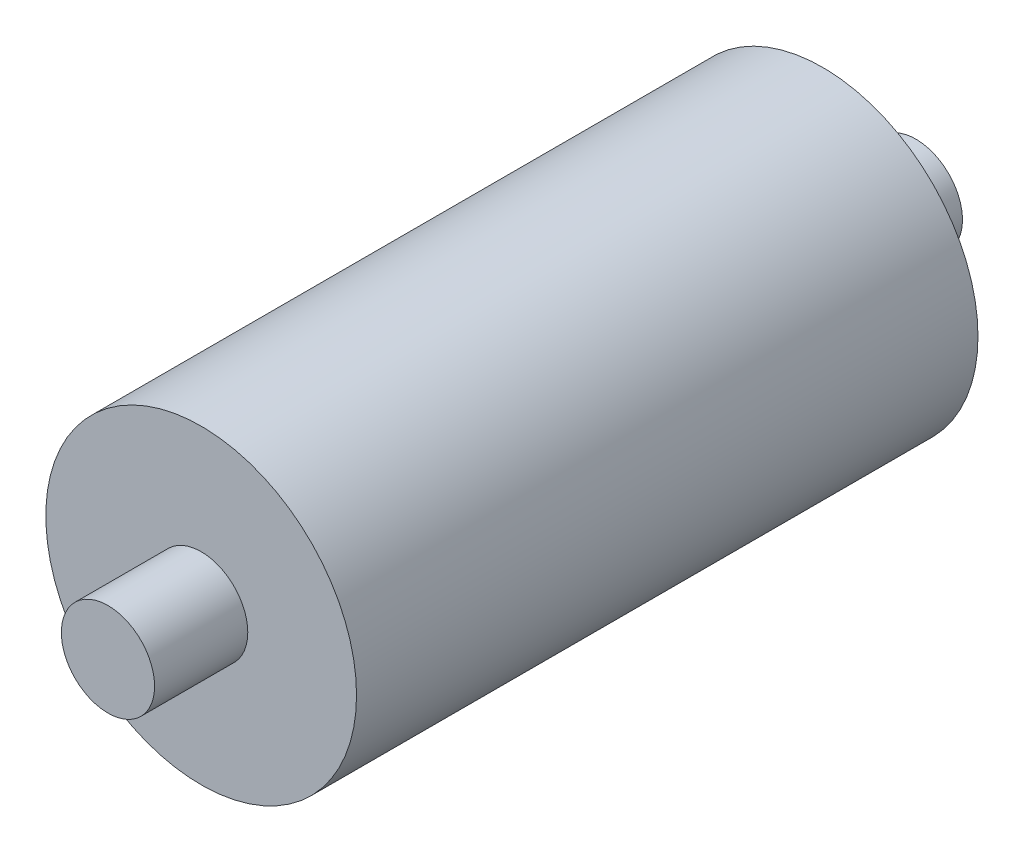
from build123d import *

# Parameters (mm, degrees)
SKETCH_1_R      = 25
EXTRUDE_1_DEPTH = 100
SKETCH_2_R      = 7.5
EXTRUDE_2_DEPTH = 15
EXTRUDE_START   = 15
SKETCH_3_R      = 7.5
EXTRUDE_3_DEPTH = 15


with BuildPart() as part:
    # 草图1 → 凸台-拉伸1 (new body)
    with BuildSketch(Plane.XY):
        Circle(SKETCH_1_R)
    extrude(amount=EXTRUDE_1_DEPTH)

    # 草图2 → 凸台-拉伸2 (add)
    with BuildSketch(Plane.XY.offset(100)):
        Circle(SKETCH_2_R)
    extrude(amount=EXTRUDE_2_DEPTH)

    # 草图3 → 凸台-拉伸3 (add)
    with BuildSketch(Plane(origin=(0, 0, 0), x_dir=(-1, 0, 0), z_dir=(0, 0, -1)).offset(EXTRUDE_START)):
        with Locations(Location((0, 0, 0), (0, 0, 180))):
            Circle(SKETCH_3_R)
    extrude(amount=-EXTRUDE_3_DEPTH)


solid = part.part
